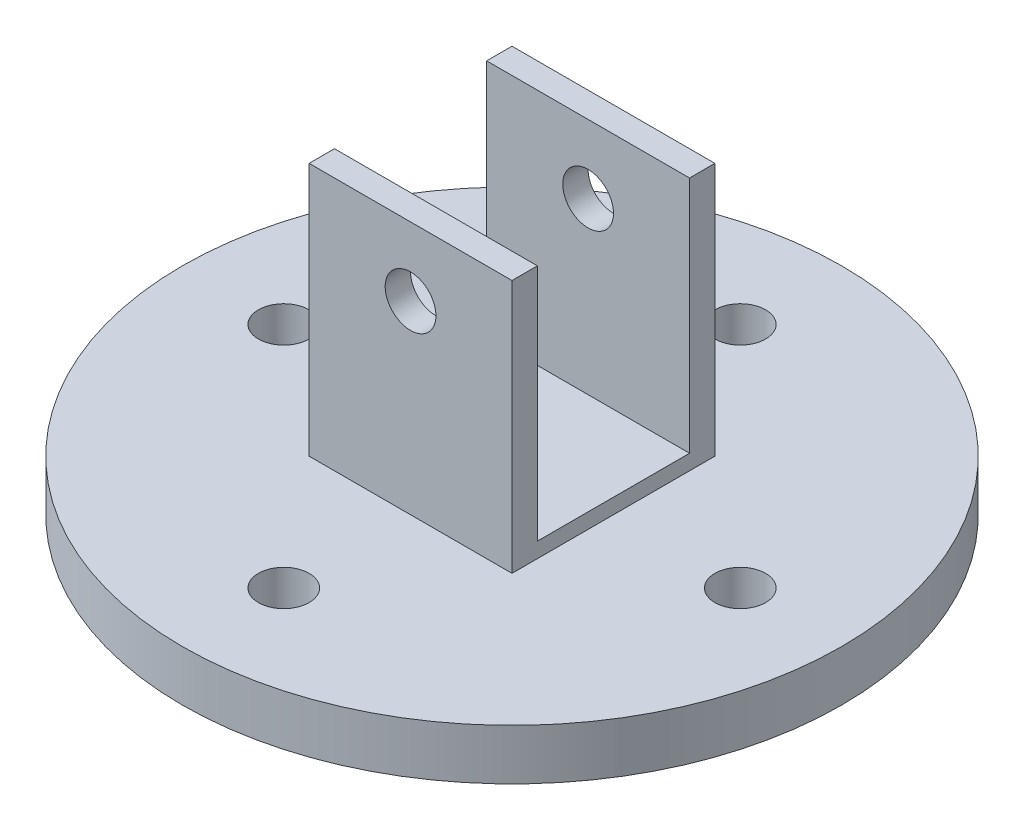
from build123d import *

# Parameters (mm, degrees)
SKETCH1_R           = 65
SKETCH1_R_2         = 15
BOSS_EXTRUDE1_DEPTH = 10
SKETCH2_R           = 5
CUT_EXTRUDE1_DEPTH  = 10
SKETCH3_W           = 40
SKETCH3_H           = 40
BOSS_EXTRUDE2_DEPTH = 50
SKETCH4_W           = 30
SKETCH4_H           = 47
CUT_EXTRUDE2_DEPTH  = 50
SKETCH5_R           = 5
CUT_EXTRUDE3_DEPTH  = 123.678441464


with BuildPart() as part:
    # Sketch1 → Boss-Extrude1 (new body)
    with BuildSketch(Plane(origin=(0, 0, 0), x_dir=(1, 0, 0), z_dir=(0, 1, 0))):
        with Locations(Location((0, 0, 0), (0, 0, 270))):
            Circle(SKETCH1_R)
        with Locations(Location((0, 0, 0), (0, 0, 270))):
            Circle(SKETCH1_R_2, mode=Mode.SUBTRACT)
    extrude(amount=BOSS_EXTRUDE1_DEPTH)

    # Sketch2 → Cut-Extrude1 (cut)
    with BuildSketch(Plane(origin=(0, 10, 0), x_dir=(1, 0, 0), z_dir=(0, 1, 0))):
        with Locations(Location((0, 45, 0), (0, 0, 270))):
            Circle(SKETCH2_R)
        with Locations(Location((45, 0, 0), (0, 0, 270))):
            Circle(SKETCH2_R)
        with Locations(Location((0, -45, 0), (0, 0, 270))):
            Circle(SKETCH2_R)
        with Locations(Location((-45, 0, 0), (0, 0, 270))):
            Circle(SKETCH2_R)
    extrude(amount=-CUT_EXTRUDE1_DEPTH, mode=Mode.SUBTRACT)

    # Sketch3 → Boss-Extrude2 (add)
    with BuildSketch(Plane(origin=(0, 10, 0), x_dir=(1, 0, 0), z_dir=(0, 1, 0))):
        Rectangle(SKETCH3_W, SKETCH3_H)
    extrude(amount=BOSS_EXTRUDE2_DEPTH)

    # Sketch4 → Cut-Extrude2 (cut)
    with BuildSketch(Plane(origin=(20, 0, 0), x_dir=(0, 0, -1), z_dir=(1, 0, 0))):
        with Locations((0, 36.5)):
            Rectangle(SKETCH4_W, SKETCH4_H)
    extrude(amount=-CUT_EXTRUDE2_DEPTH, mode=Mode.SUBTRACT)

    # Sketch5 → Cut-Extrude3 (cut, through all)
    with BuildSketch(Plane.XY.offset(20)):
        with Locations((0, 46.469084147)):
            Circle(SKETCH5_R)
    extrude(amount=-CUT_EXTRUDE3_DEPTH, mode=Mode.SUBTRACT)


solid = part.part
